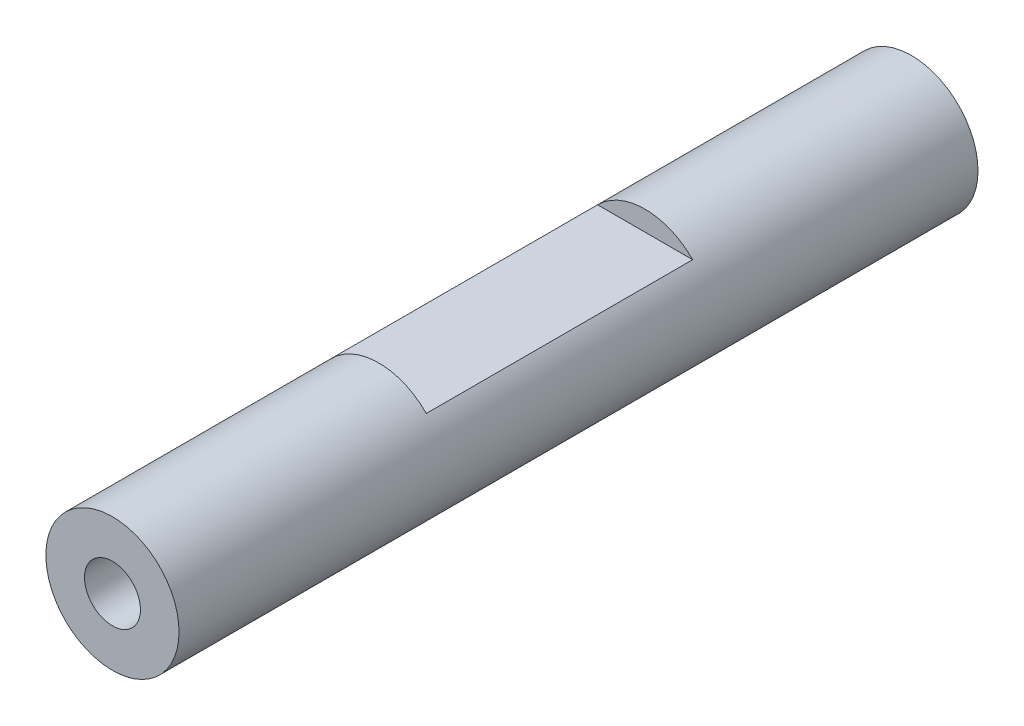
SolidWorks part; units mm, degrees
ref_plane "Front Plane" through (0, 0, 0) normal (0, 0, 1) x (1, 0, 0)
ref_plane "Top Plane" through (0, 0, 0) normal (0, 1, 0) x (1, 0, 0)
ref_plane "Right Plane" through (0, 0, 0) normal (1, 0, 0) x (0, 0, -1)
sketch "Sketch1" plane through (0, 0, 0) normal (0, 0, 1) x (1, 0, 0)
  line L1 (-90, -55) -> (90, -55) construction
  line L2 (-90, -55) -> (-90, 55) construction
  line L3 (-90, 55) -> (90, 55) construction
  line L4 (90, -55) -> (90, 55) construction
  line L5 (-90, -55) -> (90, 55) construction
  line L6 (-90, 55) -> (90, -55) construction
  circle A0 centre (-90, 55) radius 5
  point P0 (0, 0)
  dimension "D3" = 10
  dimension "D1" = 180
  dimension "D2" = 110
extrude "Boss-Extrude1" add sketch "Sketch1" along normal blind 60 contours A0
ref_plane "Plane1" through (0, 60, 0) normal (0, 1, 0) x (1, 0, 0)
sketch "Sketch2" plane through (0, 60, 0) normal (0, 1, 0) x (1, 0, 0)
  line L0 (-90, -60) -> (-90, 14.4737) construction
  line L1 (-116.9537, -30) -> (-70.7189, -30) construction
  line L2 (-95, -60) -> (-85, -60) construction
  line L3 (-85, 0) -> (-95, 0) construction
  line L5 (-100, -40) -> (-80, -40)
  line L6 (-100, -40) -> (-100, -20)
  line L7 (-100, -20) -> (-80, -20)
  line L8 (-80, -40) -> (-80, -20)
  line L9 (-100, -40) -> (-80, -20) construction
  line L10 (-100, -20) -> (-80, -40) construction
  point P9 (-90, -30)
  dimension "D1" = 30
  dimension "D2" = 20
  dimension "D3" = 20
extrude "Cut-Extrude1" cut sketch "Sketch2" against normal blind 1.5
ref_plane "Plane2" through (0, 55, 0) normal (0, 1, 0) x (1, 0, 0)
mirror "Mirror1" about plane through (0, 55, 0) normal (0, 1, 0) of "Cut-Extrude1"
hole_wizard "M5 Tapped Hole1" positions "3DSketch1" profile "Sketch3" tap size "M5" standard "GB"
sketch3d "3DSketch1"
  line L0 (-90, 55, 60) -> (-90, 55, 0) construction
  point P0 (-90, 55, 0)
  point P5 (-90, 55, 60)
sketch "Sketch3" plane through (-90, 55, 0) normal (1, 0, 0) x (0, 1, 0)
  line L0 (0, 0) -> (0, 16.2618)
  line L1 (0, 16.2618) -> (2.1, 15)
  line L2 (2.1, 15) -> (2.1, 0)
  line L5 (2.1, 0) -> (0, 0)
  line L10 (0, 16.2618) -> (-2.1, 15) construction
  line L11 (0, -6.35) -> (0, 107.95) construction
  dimension "螺纹孔钻头直径" = 4.2
  dimension "螺纹孔钻头深度" = 15
  dimension "导头角度" = 118
cosmetic thread "Cosmetic thread1" parameters "D1"=15, "D2"=5
cosmetic thread "Cosmetic thread2" parameters "D1"=15, "D2"=5
